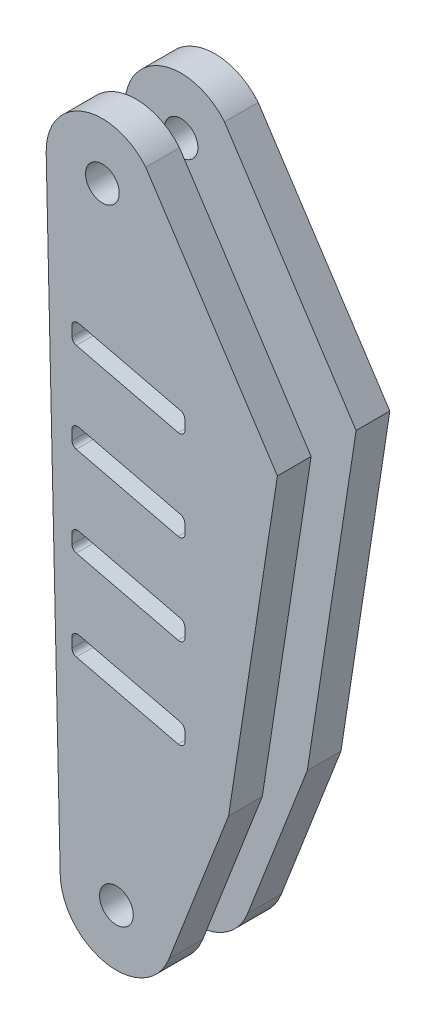
SolidWorks part; units mm, degrees
material "1060 Alloy"
ref_plane "Front Plane" through (0, 0, 0) normal (0, 0, 1) x (1, 0, 0)
ref_plane "Top Plane" through (0, 0, 0) normal (0, 1, 0) x (1, 0, 0)
ref_plane "Right Plane" through (0, 0, 0) normal (1, 0, 0) x (0, 0, -1)
sketch "Sketch1" plane through (0, 0, 0) normal (0, 0, 1) x (1, 0, 0)
  line L0 (-76.7969, 30.8379) -> (-74.2996, -79.1338)
  line L1 (-59.0785, 37.4201) -> (-35.6647, 1.5734)
  line L2 (-35.6647, 1.5734) -> (-44.3426, -55.1429)
  line L3 (-44.3426, -55.1429) -> (-54.9752, -82.5271)
  circle A0 centre (-66.7994, 31.0649) radius 3
  circle A1 centre (-64.2996, -78.9067) radius 3
  arc A2 (-59.0785, 37.4201) -> (-76.7969, 30.8379) centre (-66.7994, 31.0649) ccw
  arc A3 (-74.2996, -79.1338) -> (-54.9752, -82.5271) centre (-64.2996, -78.9067) ccw
  dimension "D3" = 6
  dimension "D4" = 6
  dimension "D7" = 10
  dimension "D1" = 110
  dimension "D2" = 10
  dimension "D5" = 10
  dimension "D6" = 10
extrude "Boss-Extrude1" add sketch "Sketch1" along normal blind 20
sketch "Sketch2" plane through (0, 0, 0) normal (0, 1, 0) x (1, 0, 0)
  line L0 (-76.7994, 0) -> (-76.7994, -20) construction
  line L1 (-111.7994, -6) -> (-41.7994, -6)
  line L2 (-111.7994, -6) -> (-111.7994, -14)
  line L3 (-111.7994, -14) -> (-41.7994, -14)
  line L4 (-41.7994, -6) -> (-41.7994, -14)
  line L5 (-111.7994, -6) -> (-41.7994, -14) construction
  line L6 (-111.7994, -14) -> (-41.7994, -6) construction
  point P0 (-76.7994, -10)
  dimension "D1" = 8
  dimension "D2" = 70
extrude "Cut-Extrude1" cut sketch "Sketch2" along normal blind 60
sketch "Sketch3" plane through (0, 0, 0) normal (0, 1, 0) x (1, 0, 0)
  line L0 (-35.6647, -20) -> (-35.6647, 0) construction
  line L1 (-13.6647, -6) -> (-57.6647, -6)
  line L2 (-13.6647, -6) -> (-13.6647, -14)
  line L3 (-13.6647, -14) -> (-57.6647, -14)
  line L4 (-57.6647, -6) -> (-57.6647, -14)
  line L5 (-13.6647, -6) -> (-57.6647, -14) construction
  line L6 (-13.6647, -14) -> (-57.6647, -6) construction
  point P0 (-35.6647, -10)
  dimension "D1" = 8
  dimension "D2" = 44
extrude "Cut-Extrude2" cut sketch "Sketch3" against normal blind 120 and the other way blind 71
sketch "Sketch4" plane through (0, 0, 0) normal (0, 1, 0) x (1, 0, 0)
  line L0 (-74.2996, -20) -> (-74.2996, 0) construction
  line L1 (-90.9345, -14) -> (-57.6647, -14)
  line L2 (-90.9345, -14) -> (-90.9345, -6)
  line L3 (-90.9345, -6) -> (-57.6647, -6)
  line L4 (-57.6647, -14) -> (-57.6647, -6)
  line L5 (-90.9345, -14) -> (-57.6647, -6) construction
  line L6 (-90.9345, -6) -> (-57.6647, -14) construction
  line L7 (-57.6647, -14) -> (-57.6647, -6) construction
  point P0 (-74.2996, -10)
  dimension "D1" = 8
extrude "Cut-Extrude3" cut sketch "Sketch4" against normal blind 120 from offset 60 offset against normal yes
fillet "Fillet1" radius 3 4 edges at (-57.6647, -60, 10) (-74.7341, -60, 10) (-76.0966, 0, 10) (-57.6647, 0, 10)
sketch "Sketch5" plane through (-76.0574, -1.7271, 0) normal (-0.9997, -0.0227, 0) x (0, 0, 1)
  line L0 (20, 32.5734) -> (20, -77.4266) construction
  line L1 (4, -7.84) -> (16, -7.84)
  line L2 (4, -7.84) -> (4, -47.84)
  line L3 (4, -47.84) -> (16, -47.84)
  line L4 (16, -7.84) -> (16, -47.84)
  line L5 (4, -7.84) -> (16, -47.84) construction
  line L6 (4, -47.84) -> (16, -7.84) construction
  point P0 (10, -27.84)
  dimension "D1" = 40
  dimension "D2" = 12
  dimension "D3" = 4
extrude "Boss-Extrude2" add sketch "Sketch5" along normal blind 3
scale "Scale1" scale about origin uniform scaling yes scale factor 0.5
sketch "Sketch6" plane through (0, 0, 8) normal (0, 0, 1) x (1, 0, 0)
  line L0 (-39.4393, -4.8166) -> (-39.1836, -5.0723)
  line L1 (-39.1836, -5.0723) -> (-39.4279, -5.3166)
  line L2 (-38.9853, -24.8115) -> (-39.4393, -4.8166) construction
  line L3 (-39.4279, -5.3166) -> (-39.4393, -4.8166)
  dimension "D1" = 0.5
extrude "Cut-Extrude4" cut sketch "Sketch6" against normal blind 10
pattern_linear "LPattern1" count 40 spacing 0.5 along (0.0227, -0.9997, 0) of "Cut-Extrude4"
sketch "Sketch7" plane through (0, 0, 10) normal (0, 0, 1) x (1, 0, 0)
  line L0 (-38.1937, 6.4036) -> (-38.0575, 0.4036) construction
  line L1 (-38.3984, 15.4189) -> (-37.1498, -39.5669) construction
  line L2 (-38.0575, 0.4036) -> (-23.9769, -2.9856) construction
  line L3 (-23.9769, -2.9856) -> (-24.1131, 3.0144) construction
  line L4 (-24.1131, 3.0144) -> (-38.1937, 6.4036) construction
  line L5 (-26.0777, 1.4302) -> (-36.1352, 3.851)
  line L6 (-36.1352, 3.851) -> (-36.0929, 1.9879)
  line L7 (-36.0929, 1.9879) -> (-26.0354, -0.433)
  line L8 (-26.0354, -0.433) -> (-26.0777, 1.4302)
  line L9 (-26.0777, -6.5698) -> (-36.1352, -4.149)
  line L10 (-36.1352, -4.149) -> (-36.0929, -6.0121)
  line L11 (-36.0929, -6.0121) -> (-26.0354, -8.433)
  line L12 (-26.0354, -8.433) -> (-26.0777, -6.5698)
  line L13 (-26.0777, -14.5698) -> (-36.1352, -12.149)
  line L14 (-36.1352, -12.149) -> (-36.0929, -14.0121)
  line L15 (-36.0929, -14.0121) -> (-26.0354, -16.433)
  line L16 (-26.0354, -16.433) -> (-26.0777, -14.5698)
  line L17 (-26.0777, -22.5698) -> (-36.1352, -20.149)
  line L18 (-36.1352, -20.149) -> (-36.0929, -22.0121)
  line L19 (-36.0929, -22.0121) -> (-26.0354, -24.433)
  line L20 (-26.0354, -24.433) -> (-26.0777, -22.5698)
  dimension "D1" = 6
  dimension "D2" = 14
  dimension "D3" = 2
  dimension "D4" = 4
extrude "Cut-Extrude6" cut sketch "Sketch7" against normal blind 10
fillet "Fillet3" radius 0.5 32 edges at (-28.8323, -23.7598, 5) (-28.8323, -21.9068, 5) (-28.8323, -15.7598, 5) (-28.8323, -13.9068, 5) (-28.8323, -7.7598, 5) (-28.8323, -5.9068, 5) (-26.0354, -24.433, 8.5) (-26.0777, -22.5698, 8.5) (-26.0354, -16.433, 8.5) (-26.0777, -14.5698, 8.5) (-26.0354, -8.433, 8.5) (-26.0777, -6.5698, 8.5) (-26.0354, -24.433, 1.5) (-26.0777, -22.5698, 1.5) (-26.0354, -16.433, 1.5) (-26.0777, -14.5698, 1.5) (-26.0354, -8.433, 1.5) (-26.0777, -6.5698, 1.5) (-36.0929, 1.9879, 1.5) (-36.1352, 3.851, 1.5) (-26.0354, -0.433, 1.5) (-26.0777, 1.4302, 1.5) (-36.0929, -22.0121, 5) (-36.1352, -20.149, 5) (-36.0929, -14.0121, 5) (-36.1352, -12.149, 5) (-36.0929, -6.0121, 5) (-36.1352, -4.149, 5) (-26.0354, -0.433, 8.5) (-26.0777, 1.4302, 8.5) (-36.1352, 3.851, 8.5) (-36.0929, 1.9879, 8.5)
